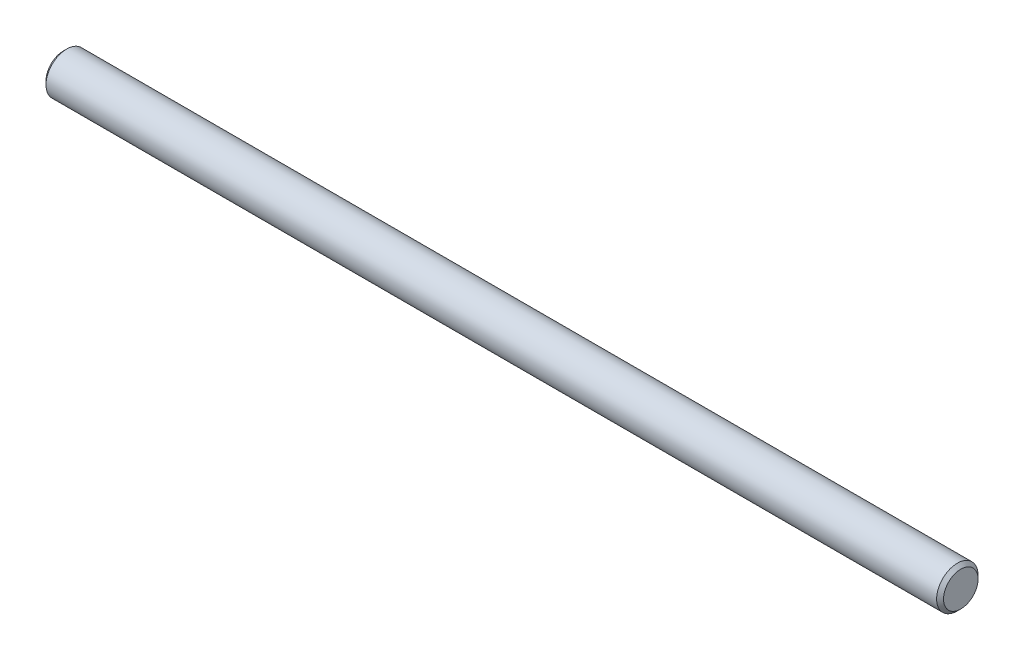
SolidWorks part; units mm, degrees
material "镀铬光轴"
ref_plane "Front Plane" through (0, 0, 0) normal (0, 0, 1) x (1, 0, 0)
ref_plane "Top Plane" through (0, 0, 0) normal (0, 1, 0) x (1, 0, 0)
ref_plane "Right Plane" through (0, 0, 0) normal (1, 0, 0) x (0, 0, -1)
sketch "Sketch1" plane through (0, 0, 0) normal (0, 0, 1) x (1, 0, 0)
  line L0 (0, 0) -> (59.0007, 0) construction
  line L2 (0, 0) -> (130, 0)
  line L3 (0, 0) -> (0, 3)
  line L4 (0, 3) -> (130, 3)
  line L5 (130, 0) -> (130, 3)
  dimension "D1" = 3
  dimension "D2" = 130
revolve "Revolve1" add sketch "Sketch1" angle 360 about L0
chamfer "Chamfer1" distance 0.5 angle 45 2 edges at (130, 0, 3) (0, 0, 3)
